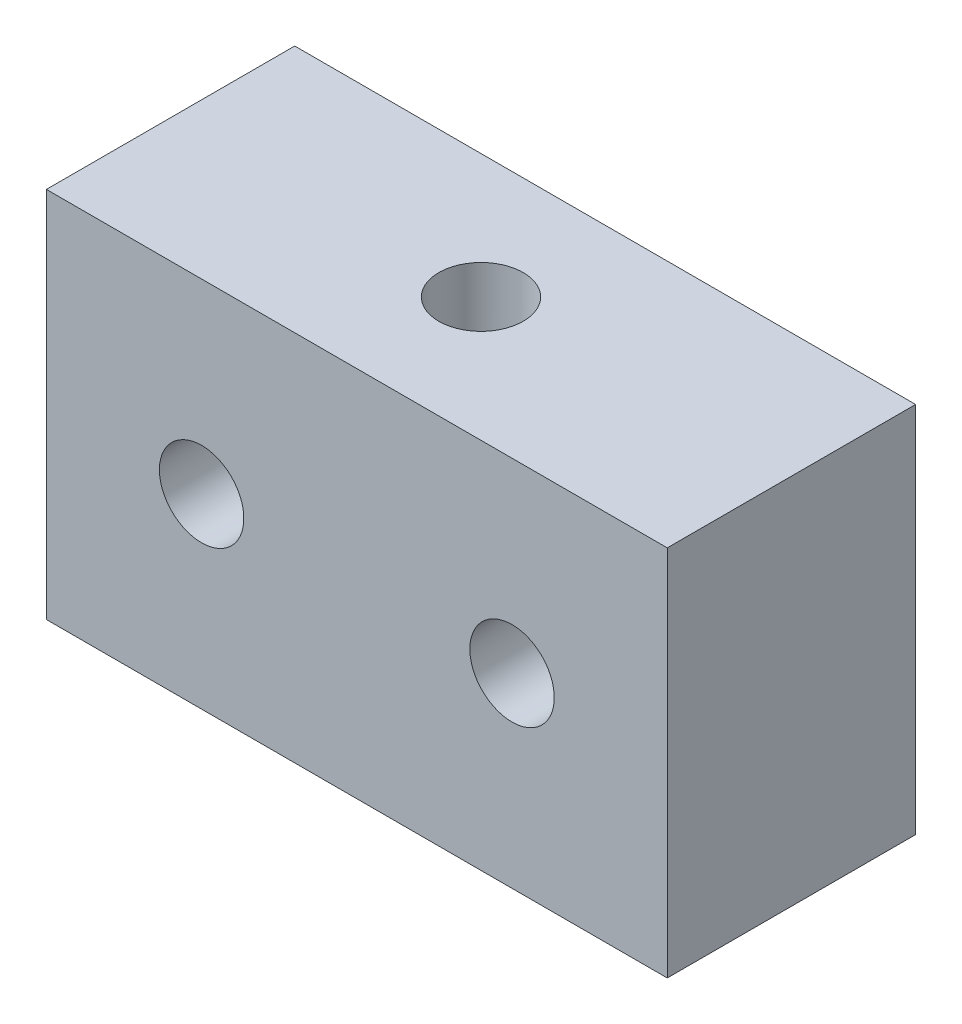
SolidWorks part; units mm, degrees
ref_plane "Front Plane" through (0, 0, 0) normal (0, 0, 1) x (1, 0, 0)
ref_plane "Top Plane" through (0, 0, 0) normal (0, 1, 0) x (1, 0, 0)
ref_plane "Right Plane" through (0, 0, 0) normal (1, 0, 0) x (0, 0, -1)
other "Configuration Table"
sketch "Sketch1" plane through (0, 0, 0) normal (0, 0, 1) x (1, 0, 0)
  line L1 (0, 0) -> (50, 0)
  line L2 (0, 0) -> (0, -30)
  line L3 (0, -30) -> (50, -30)
  line L4 (50, 0) -> (50, -30)
  dimension "D1" = 50
  dimension "D2" = 30
extrude "Boss-Extrude1" add sketch "Sketch1" along normal blind 20
sketch "Sketch2" plane through (0, 0, 0) normal (0, 0, -1) x (-1, 0, 0)
  line L0 (-25, 0) -> (-25, -30) construction
  line L1 (-50, 0) -> (0, 0) construction
  line L2 (0, -30) -> (-50, -30) construction
  circle A0 centre (-37.5, -15) radius 2.4919
  circle A1 centre (-12.5, -15) radius 2.4919
  point P6 (-37.5, -15)
  point P8 (-12.5, -15)
  dimension "D1" = 25
hole_wizard "M8 Tapped Hole1" positions "Sketch2" profile "Sketch3" tap size "M8" standard "GB" end condition through all
sketch "Sketch3" plane through (12.5, -15, 0) normal (1, 0, 0) x (0, 1, 0)
  line L0 (0, 0) -> (0, 20)
  line L1 (0, 20) -> (3.4, 20)
  line L2 (3.4, 20) -> (3.4, 0)
  line L5 (3.4, 0) -> (0, 0)
  line L11 (0, -6.35) -> (0, 107.95) construction
  dimension "通孔螺纹孔钻头直径" = 6.8
  dimension "通孔螺纹孔钻头深度" = 20
cosmetic thread "CosmeticThread hole thread line 1" parameters "D2"=8
cosmetic thread "CosmeticThread hole thread line 2" parameters "D2"=8
sketch "Sketch4" plane through (0, 0, 0) normal (0, 1, 0) x (1, 0, 0)
  line L0 (0, -10) -> (50, -10) construction
  line L1 (0, -20) -> (0, 0) construction
  line L2 (50, -20) -> (50, 0) construction
  line L3 (25, 0) -> (25, -20) construction
  line L4 (50, 0) -> (0, 0) construction
  line L5 (50, -20) -> (0, -20) construction
  circle A0 centre (25, -10) radius 4
  dimension "D1" = 8
hole_wizard "M8 Tapped Hole2" positions "3DSketch1" profile "Sketch5" tap size "M8" standard "GB" end condition through all
sketch3d "3DSketch1"
  point P0 (25, 0, 10)
cosmetic thread "CosmeticThread hole thread line 3" parameters "D1"=10, "D2"=8
sketch "Sketch5" plane through (25, 0, 10) normal (1, 0, 0) x (0, 0, 1)
  line L0 (0, 0) -> (0, 30)
  line L1 (0, 30) -> (3.4, 30)
  line L2 (3.4, 30) -> (3.4, 0)
  line L5 (3.4, 0) -> (0, 0)
  line L11 (0, -6.35) -> (0, 107.95) construction
  dimension "通孔螺纹孔钻头直径" = 6.8
  dimension "通孔螺纹孔钻头深度" = 30
sketch "Sketch6" plane through (0, -30, 0) normal (0, -1, 0) x (1, 0, 0)
  line L0 (25, 0) -> (25, 20) construction
  circle A0 centre (25, 10) radius 4
extrude "Cut-Extrude1" cut sketch "Sketch6" against normal blind 20
